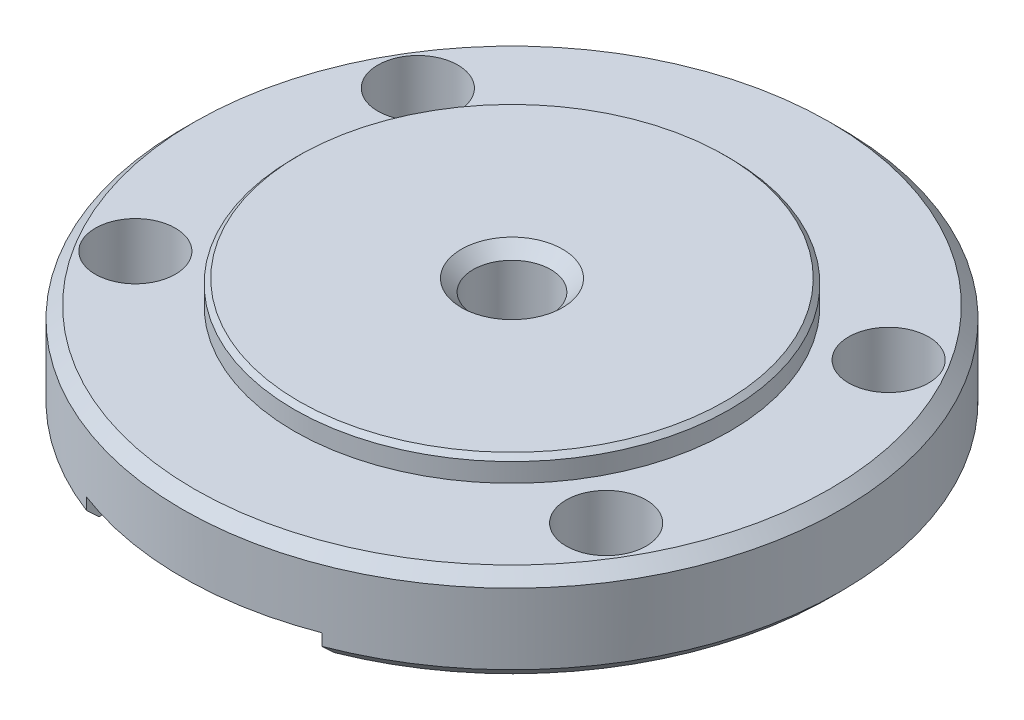
from build123d import *

# Parameters (mm, degrees)
SKETCH1_W            = 14
SKETCH1_H            = 5
SKETCH3_OUTSIDE_W    = 37.982
SKETCH3_OUTSIDE_H    = 37.982
SKETCH3_OUTSIDE_R    = 9.25
CUT_EXTRUDE2_DEPTH   = 1
M3_CLEARANCE_HOLE1_D = 3.4
SKETCH6_W            = 10
SKETCH6_H            = 31.428384658
CUT_EXTRUDE3_DEPTH   = 1
M4_TAPPED_HOLE1_D    = 3.3
CHAMFER1_SIZE        = 0.5
CHAMFER2_SIZE        = 0.2


with BuildPart() as part:
    # Sketch1 → Revolve1 (revolve)
    with BuildSketch(Plane.XY, mode=Mode.PRIVATE) as revolve1_sk:
        with Locations((7, 2.5)):
            Rectangle(SKETCH1_W, SKETCH1_H)
    revolve(revolve1_sk.sketch.rotate(Axis((0, 0, 0), (0, 1, 0)), 90), axis=Axis((0, 0, 0), (0, 1, 0)))

    # Sketch3 outside → Cut-Extrude2 (cut)
    with BuildSketch(Plane(origin=(0, 5, 0), x_dir=(1, 0, 0), z_dir=(0, 1, 0))):
        Rectangle(SKETCH3_OUTSIDE_W, SKETCH3_OUTSIDE_H)
        with Locations(Location((0, 0, 0), (0, 0, 270))):
            Circle(SKETCH3_OUTSIDE_R, mode=Mode.SUBTRACT)
    extrude(amount=-CUT_EXTRUDE2_DEPTH, mode=Mode.SUBTRACT)

    # M3 Clearance Hole1 (through all)
    with Locations(Plane(origin=(0, 0, 0), x_dir=(-1, 0, 0), z_dir=(0, -1, 0))):
        with Locations((10, -6), (10, 6), (-10, -6), (-10, 6)):
            Hole(M3_CLEARANCE_HOLE1_D / 2)

    # Sketch6 → Cut-Extrude3 (cut)
    with BuildSketch(Plane.XZ):
        Rectangle(SKETCH6_W, SKETCH6_H)
    extrude(amount=-CUT_EXTRUDE3_DEPTH, mode=Mode.SUBTRACT)

    # M4 Tapped Hole1 (through all)
    with Locations(Plane(origin=(0, 1, 0), x_dir=(-1, 0, 0), z_dir=(0, -1, 0))):
        with Locations((0, 0)):
            Hole(M4_TAPPED_HOLE1_D / 2)

    # Chamfer1
    chamfer1_edges = [part.edges().sort_by_distance(p)[0] for p in [
        (0, 4, 14),
        (14, 0, 0),
        (-14, 0, 0),
        (-1.65, 1, 0),
        (-1.65, 5, 0),
    ]]
    chamfer(chamfer1_edges, length=CHAMFER1_SIZE)

    # Chamfer2
    chamfer2_edges = [part.edges().sort_by_distance(p)[0] for p in [
        (0, 5, -9.25),
    ]]
    chamfer(chamfer2_edges, length=CHAMFER2_SIZE)


solid = part.part
